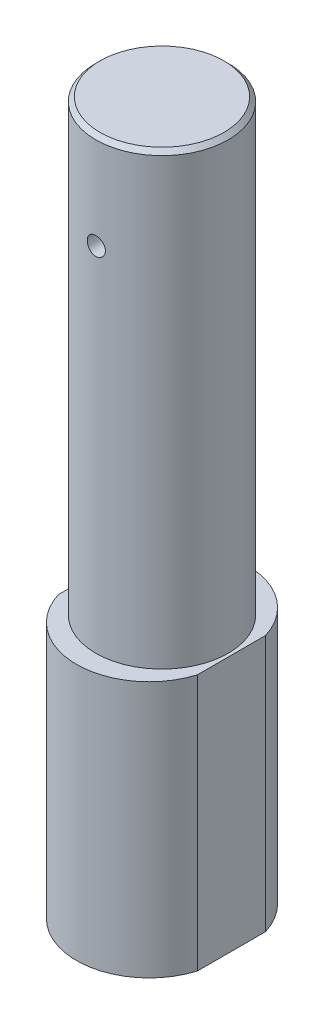
SolidWorks part; units mm, degrees
material "45"
ref_plane "前视基准面" through (0, 0, 0) normal (0, 0, 1) x (1, 0, 0)
ref_plane "上视基准面" through (0, 0, 0) normal (0, 1, 0) x (1, 0, 0)
ref_plane "右视基准面" through (0, 0, 0) normal (1, 0, 0) x (0, 0, -1)
sketch "草图1" plane through (0, 0, 0) normal (0, 1, 0) x (1, 0, 0)
  line L0 (0, 6) -> (0, -6) construction
  line L5 (0, 0) -> (32.5, 0) construction
  line L6 (32.5, -15.9875) -> (32.5, 15.9875)
  line L7 (-32.5, -15.9875) -> (-32.5, 15.9875)
  arc A0 (32.5, 15.9875) -> (-32.5, 15.9875) centre (0, 6) ccw
  arc A1 (32.5, -15.9875) -> (-32.5, -15.9875) centre (0, -6) cw
  point P4 (0, 40)
  point P11 (-32.5, 0)
  point P12 (0, -40)
  dimension "D1" = 68
  dimension "D2" = 32.5
  dimension "D3" = 6
  dimension "D4" = 80
extrude "凸台-拉伸1" add sketch "草图1" along normal blind 120
sketch "草图2" plane through (0, 120, 0) normal (0, 1, 0) x (1, 0, 0)
  circle A0 centre (0, 0) radius 31
  dimension "D1" = 62
extrude "凸台-拉伸2" add sketch "草图2" along normal blind 210
ref_plane "基准面1" through (0, 0, 31) normal (0, 0, 1) x (1, 0, 0)
hole_wizard "M10 螺纹孔1" positions "草图3" profile "草图4" tap size "M10" standard "GB"
sketch "草图3" plane through (0, 0, 31) normal (0, 0, 1) x (1, 0, 0)
  line L0 (32.5, 120) -> (-32.5, 120) construction
  point P0 (0, 285)
  dimension "D1" = 165
sketch "草图4" plane through (0, 285, 31) normal (1, 0, 0) x (0, -1, 0)
  line L0 (0, 0) -> (0, 30.0537)
  line L1 (0, 30.0537) -> (4.25, 27.5)
  line L2 (4.25, 27.5) -> (4.25, 0)
  line L5 (4.25, 0) -> (0, 0)
  line L10 (0, 30.0537) -> (-4.25, 27.5) construction
  line L11 (0, -6.35) -> (0, 107.95) construction
  dimension "螺纹孔钻头直径" = 8.5
  dimension "螺纹孔钻头深度" = 27.5
  dimension "导头角度" = 118
cosmetic thread "孔螺蚊线1"
chamfer "倒角1" distance 2 angle 45 1 edges at (0, 330, 31)
